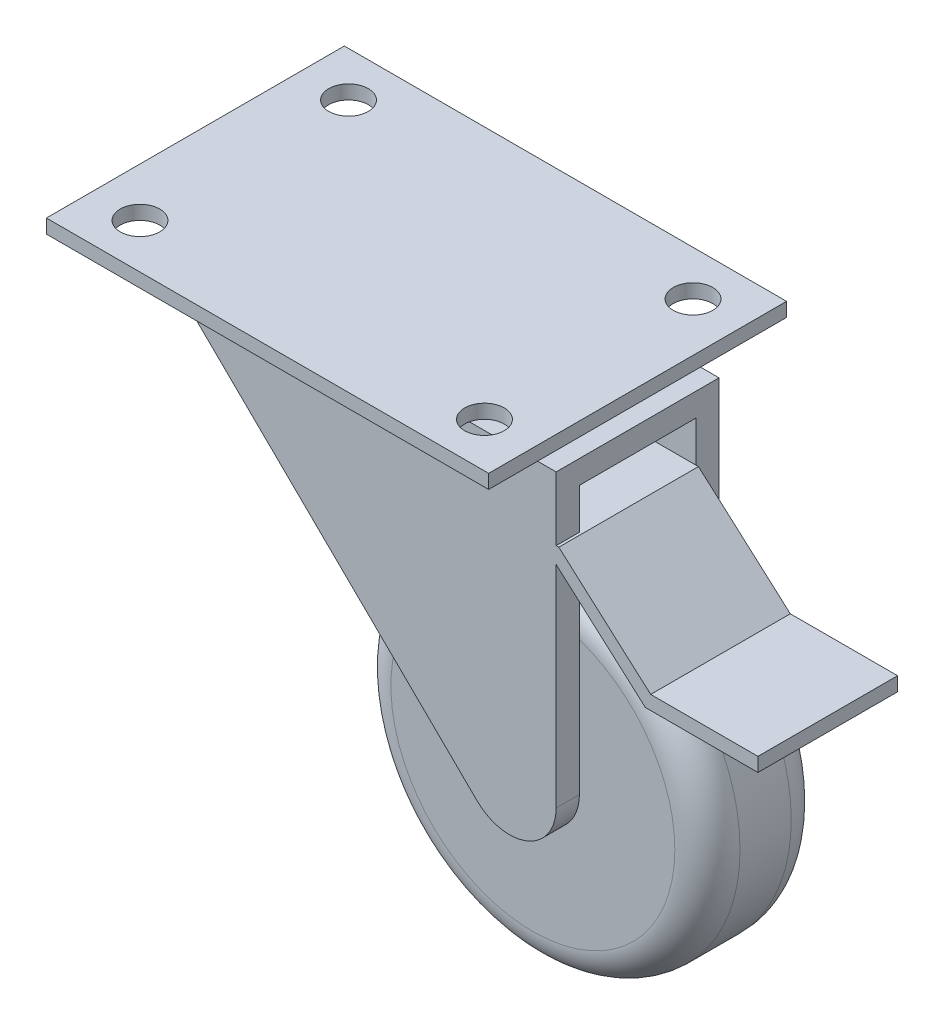
SolidWorks part; units mm, degrees
ref_plane "前视基准面" through (0, 0, 0) normal (0, 0, 1) x (1, 0, 0)
ref_plane "上视基准面" through (0, 0, 0) normal (0, 1, 0) x (1, 0, 0)
ref_plane "右视基准面" through (0, 0, 0) normal (1, 0, 0) x (0, 0, -1)
sketch "草图1" plane through (0, 0, 0) normal (0, 0, 1) x (1, 0, 0)
  circle A0 centre (0, 0) radius 37.5
  dimension "D1" = 75
extrude "凸台-拉伸1" add sketch "草图1" along normal mid plane 25
fillet "圆角1" radius 7 2 edges at (37.5, 0, -12.5) (37.5, 0, 12.5)
sketch "草图2" plane through (0, 0, 0) normal (0, 0, 1) x (1, 0, 0)
  circle A0 centre (0, 0) radius 5.4118
extrude "凸台-拉伸2" add sketch "草图2" along normal mid plane 30
sketch "草图3" plane through (0, 0, 12.5) normal (0, 0, 1) x (1, 0, 0)
  line L0 (-7.0087, -7.1329) -> (-85, 69.5)
  line L1 (-85, 69.5) -> (10, 69.5)
  line L2 (10, 69.5) -> (10, 0)
  line L3 (0, 0) -> (32.4824, 0) construction
  arc A0 (-7.0087, -7.1329) -> (10, 0) centre (0, 0) ccw
  circle A1 centre (0, 0) radius 37.5 construction
  dimension "D2" = 10
  dimension "D1" = 107
  dimension "D3" = 95
  dimension "D4" = 90
extrude "凸台-拉伸3" add sketch "草图3" along normal blind 5
mirror "镜向1" about plane through (0, 0, 0) normal (0, 0, 1) of "凸台-拉伸3"
sketch "草图4" plane through (0, 69.5, 0) normal (0, 1, 0) x (1, 0, 0)
  line L0 (-85, 0) -> (0, 0) construction
  line L1 (-85, 32) -> (10, 32)
  line L2 (-85, 32) -> (-85, -32)
  line L3 (-85, -32) -> (10, -32)
  line L4 (10, 32) -> (10, -32)
  line L5 (-85, 17.5) -> (-85, 12.5) construction
  dimension "D1" = 95
  dimension "D2" = 64
extrude "凸台-拉伸4" add sketch "草图4" against normal blind 3
sketch "草图6" plane through (0, 69.5, 0) normal (0, 1, 0) x (1, 0, 0)
  line L0 (-37.5, 32) -> (-37.5, 42.7223) construction
  line L1 (-74.5, 22.4) -> (-0.5, 22.4) construction
  line L2 (-74.5, 22.4) -> (-74.5, -22.4) construction
  line L3 (-74.5, -22.4) -> (-0.5, -22.4) construction
  line L4 (-0.5, 22.4) -> (-0.5, -22.4) construction
  line L5 (-74.5, 22.4) -> (-0.5, -22.4) construction
  line L6 (-74.5, -22.4) -> (-0.5, 22.4) construction
  line L7 (10, 32) -> (-85, 32) construction
  circle A0 centre (-0.5, -22.4) radius 4.25
  circle A1 centre (-0.5, 22.4) radius 4.25
  circle A2 centre (-74.5, 22.4) radius 4.25
  circle A3 centre (-74.5, -22.4) radius 4.25
  point P0 (-37.5, 0)
  dimension "D3" = 8.5
  dimension "D1" = 44.8
  dimension "D2" = 74
extrude "切除-拉伸1" cut sketch "草图6" against normal through all
sketch "草图9" plane through (0, 0, 17.5) normal (0, 0, 1) x (1, 0, 0)
  line L1 (10, 66.5) -> (-82.5394, 66.5)
  line L2 (10, 66.5) -> (10, 57.5176)
  line L3 (10, 57.5176) -> (-82.5394, 57.5176)
  line L4 (-82.5394, 66.5) -> (-82.5394, 57.5176)
extrude "切除-拉伸2" cut sketch "草图9" against normal through all
sketch "草图10" plane through (0, 57.5176, 0) normal (0, 1, 0) x (1, 0, 0)
  line L1 (10, 17.5) -> (-72.8052, 17.5)
  line L2 (10, 17.5) -> (10, -17.5)
  line L3 (10, -17.5) -> (-72.8052, -17.5)
  line L4 (-72.8052, 17.5) -> (-72.8052, -17.5)
extrude "凸台-拉伸5" add sketch "草图10" along normal blind 5
sketch "草图11" plane through (0, 62.5176, 0) normal (0, 1, 0) x (1, 0, 0)
  line L0 (10, 0) -> (-72.8052, 0) construction
  line L1 (10, -32) -> (10, 32) construction
  line L2 (-72.8052, 17.5) -> (-72.8052, -17.5) construction
  line L3 (-72.8052, -17.5) -> (10, -17.5) construction
  circle A0 centre (-31.4026, 0) radius 17.5
extrude "凸台-拉伸6" add sketch "草图11" along normal up to surface (3.9824 mm away) up to face at (-37.5, 66.5, 0)
sketch "草图8" plane through (0, 0, 17.5) normal (0, 0, 1) x (1, 0, 0)
  line L0 (10, 47.292) -> (29.7342, 29.7741)
  line L1 (10, 0) -> (10, 62.5176) construction
  line L2 (29.7342, 29.7741) -> (53.3472, 29.7741)
  line L3 (10, 47.292) -> (-19.25, 47.292)
extrude "拉伸-薄壁1" add sketch "草图8" against normal up to surface (30 mm away) thin up to face at (-16.1502, 42.994, -12.5) thin type mid plane wall 3
